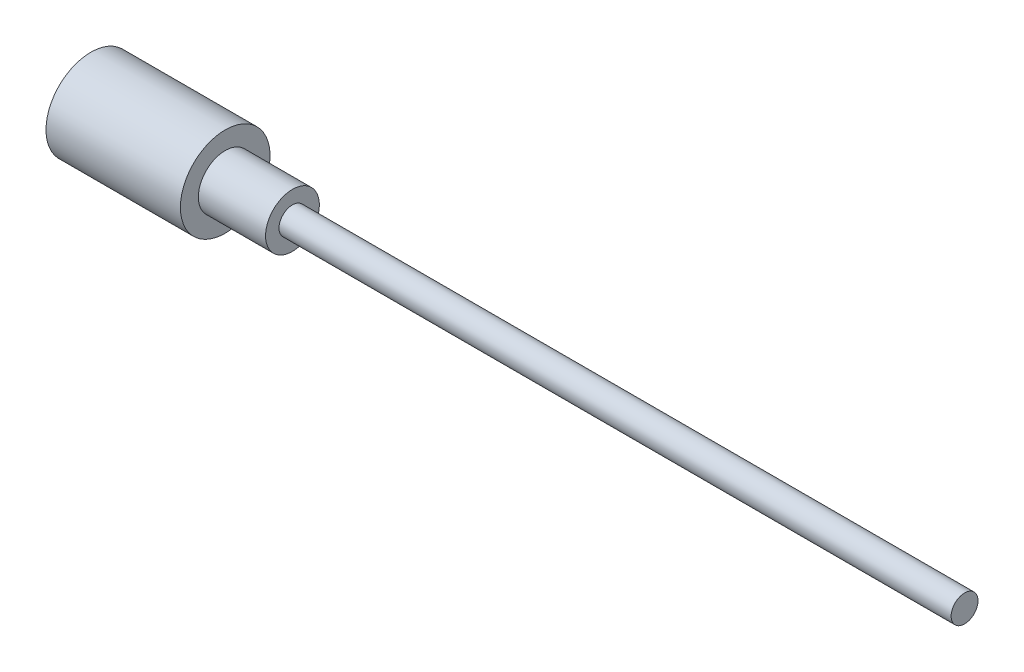
SolidWorks part; units mm, degrees
ref_plane "Front Plane" through (0, 0, 0) normal (0, 0, 1) x (1, 0, 0)
ref_plane "Top Plane" through (0, 0, 0) normal (0, 1, 0) x (1, 0, 0)
ref_plane "Right Plane" through (0, 0, 0) normal (1, 0, 0) x (0, 0, -1)
sketch "Sketch1" plane through (0, 0, 0) normal (0, 0, 1) x (1, 0, 0)
  line L0 (0, 0) -> (0, 10)
  line L1 (0, 10) -> (30, 10)
  line L2 (30, 10) -> (30, 6)
  line L3 (30, 6) -> (45, 6)
  line L4 (45, 6) -> (45, 3)
  line L5 (45, 3) -> (195, 3)
  line L6 (195, 3) -> (195, 0)
  line L7 (0, 0) -> (80.1322, 0) construction
  line L8 (0, 0) -> (195, 0)
  dimension "D1" = 6
  dimension "D2" = 10
  dimension "D3" = 3
  dimension "D4" = 30
  dimension "D5" = 15
  dimension "D6" = 150
revolve "Revolve1" add sketch "Sketch1" angle 360 about L7
